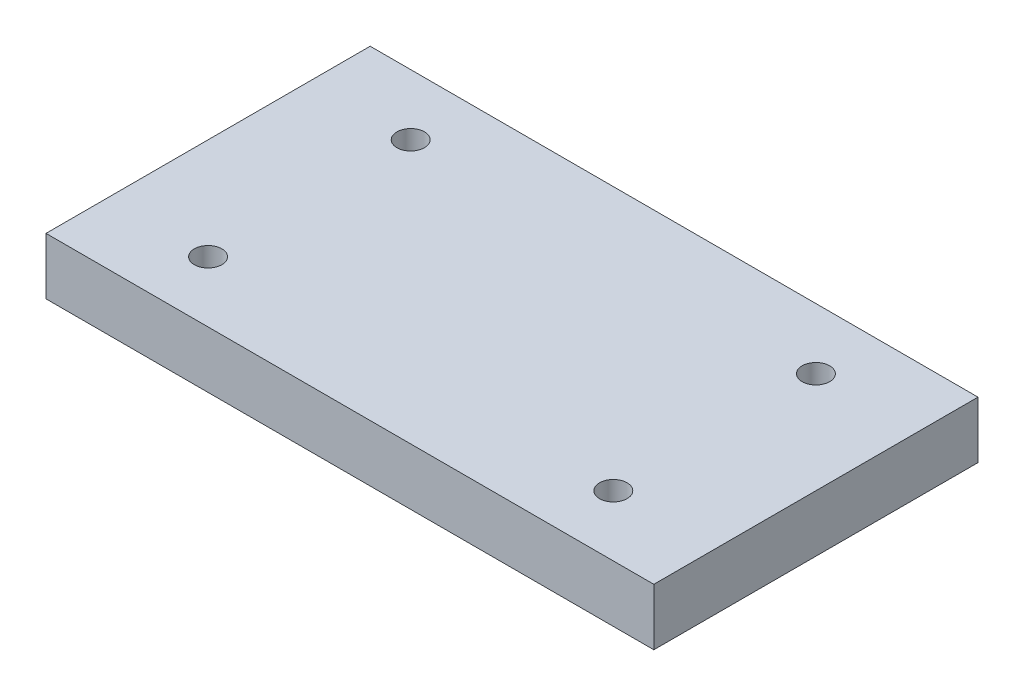
from build123d import *

# Parameters (mm, degrees)
SKETCH1_W           = 150
SKETCH1_H           = 80
BOSS_EXTRUDE1_DEPTH = 14
M8_TAPPED_HOLE1_D   = 6.8


with BuildPart() as part:
    # Sketch1 → Boss-Extrude1 (new body)
    with BuildSketch(Plane(origin=(0, 0, 0), x_dir=(1, 0, 0), z_dir=(0, 1, 0))):
        with Locations((75, 40)):
            Rectangle(SKETCH1_W, SKETCH1_H)
    extrude(amount=BOSS_EXTRUDE1_DEPTH)

    # M8 Tapped Hole1 (through all)
    with Locations(Plane(origin=(0, 14, 0), x_dir=(-1, 0, 0), z_dir=(0, 1, 0))):
        with Locations((-25, -65), (-25, -15), (-125, -15), (-125, -65)):
            Hole(M8_TAPPED_HOLE1_D / 2)


solid = part.part
